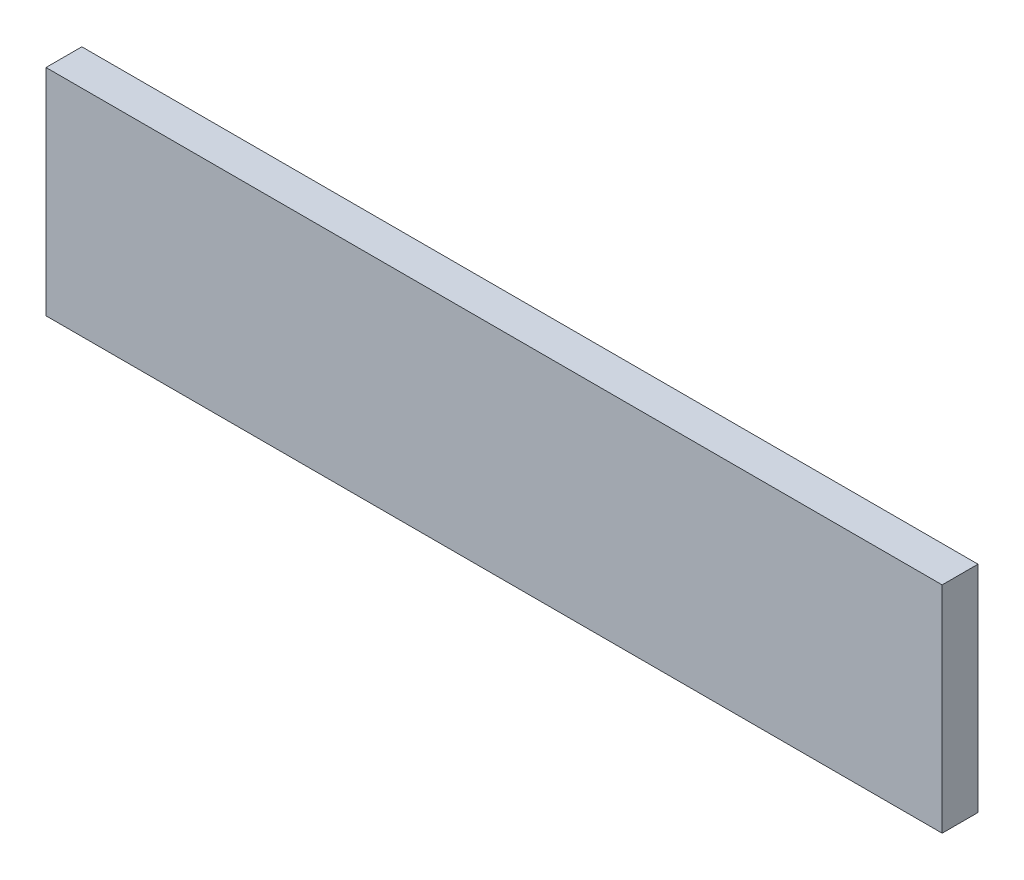
from build123d import *

# Parameters (mm, degrees)
SKETCH_1_W      = 1250
SKETCH_1_H      = 300
EXTRUDE_1_DEPTH = 50


with BuildPart() as part:
    # 草图1 → 凸台-拉伸1 (new body)
    with BuildSketch(Plane.XY):
        Rectangle(SKETCH_1_W, SKETCH_1_H)
    extrude(amount=EXTRUDE_1_DEPTH)


solid = part.part
